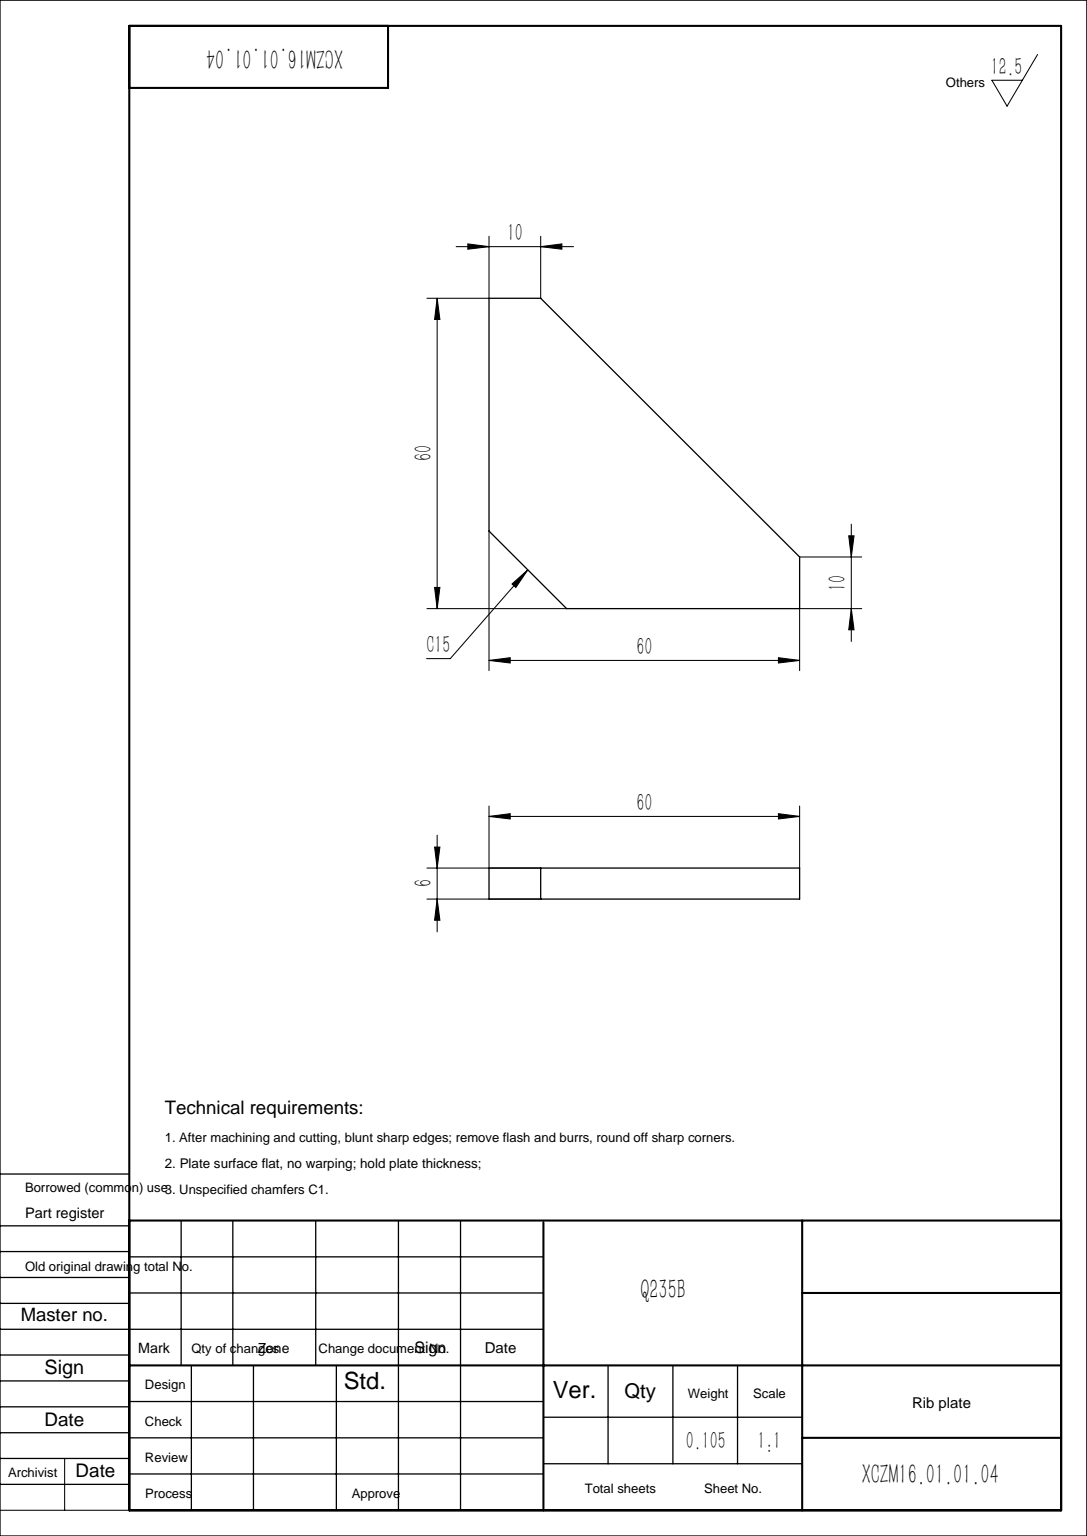
SolidWorks part; units mm, degrees
material "Q235B"
ref_plane "Front Plane" through (0, 0, 0) normal (0, 0, 1) x (1, 0, 0)
ref_plane "Top Plane" through (0, 0, 0) normal (0, 1, 0) x (1, 0, 0)
ref_plane "Right Plane" through (0, 0, 0) normal (1, 0, 0) x (0, 0, -1)
sketch "Sketch1" plane through (0, 0, 0) normal (0, 0, 1) x (1, 0, 0)
  line L0 (0, 60) -> (0, 0)
  line L1 (0, 0) -> (60, 0)
  line L2 (60, 0) -> (60, 10)
  line L3 (60, 10) -> (10, 60)
  line L4 (10, 60) -> (0, 60)
  dimension "D1" = 60
  dimension "D2" = 10
extrude "Boss-Extrude1" add sketch "Sketch1" along normal blind 6
chamfer "Chamfer1" distance 15 angle 45 1 edges at (0, 0, 3)
